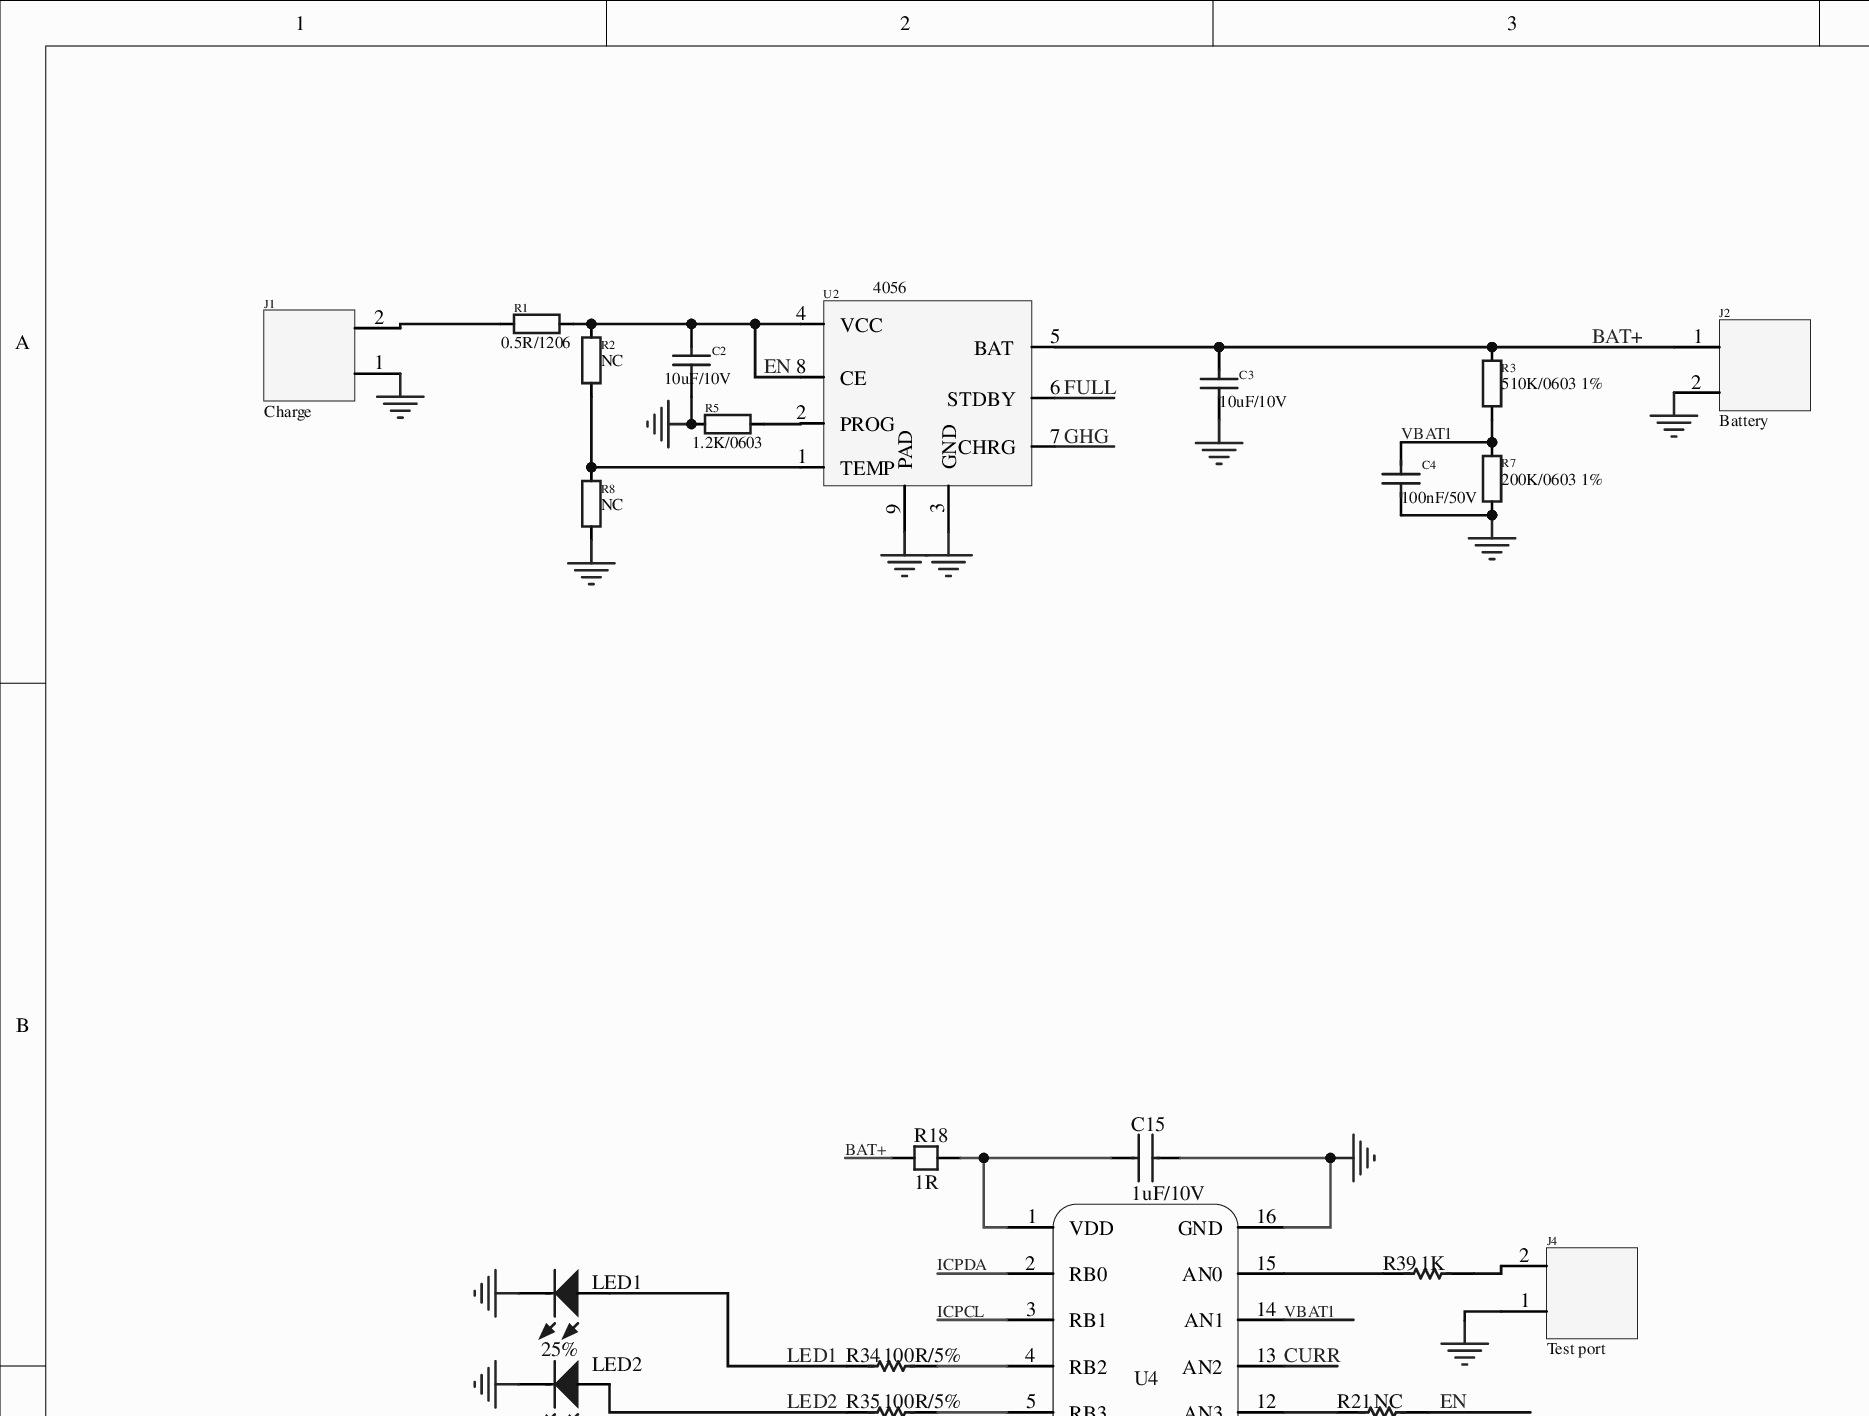
[diagram p0: MISC75737-5.SchDoc, top left]
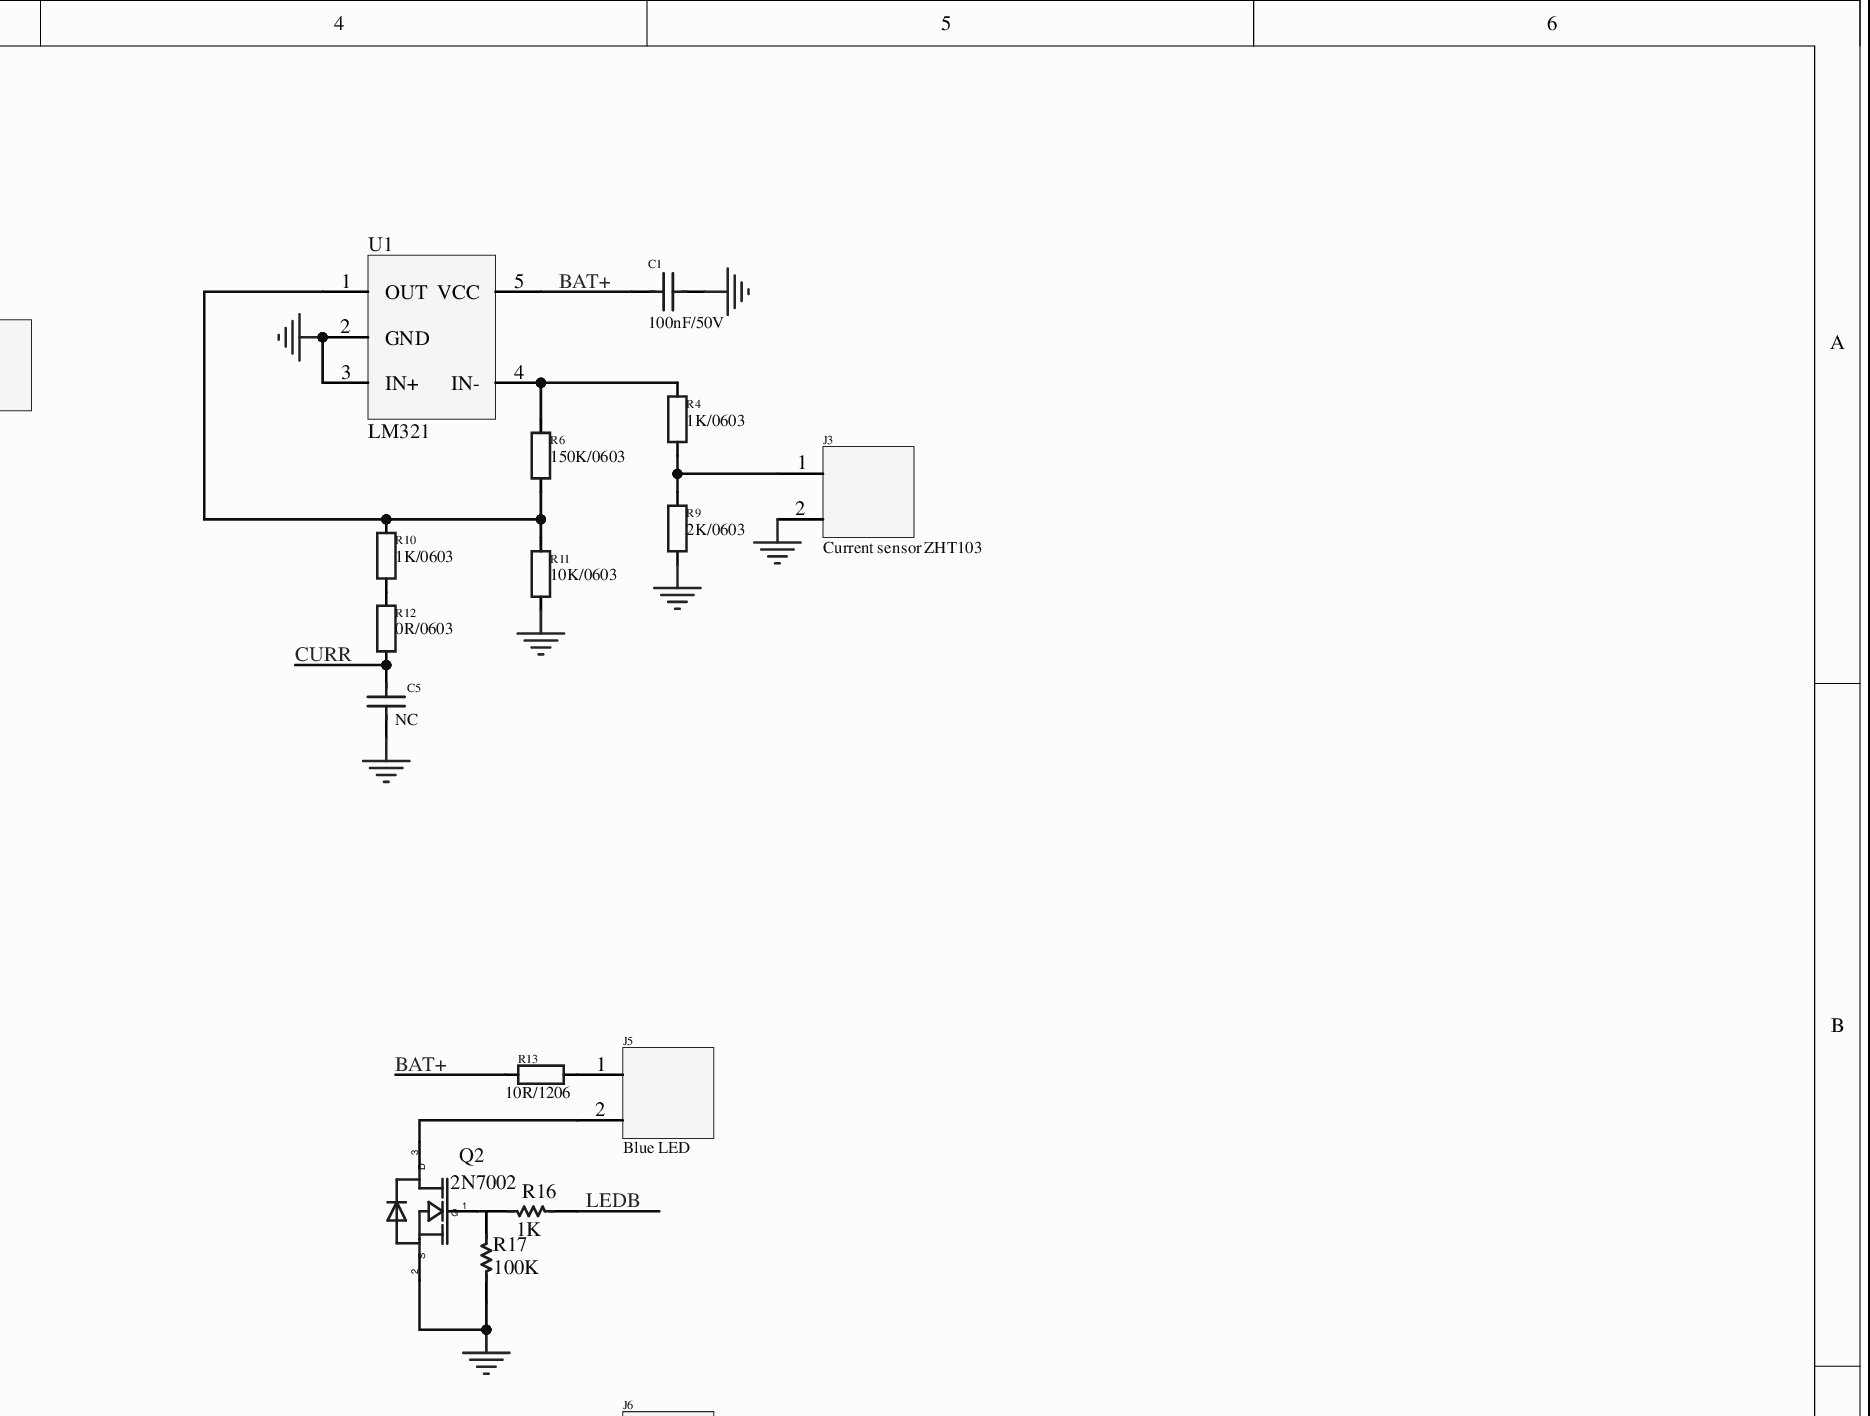
[diagram p1: MISC75737-5.SchDoc, top right]
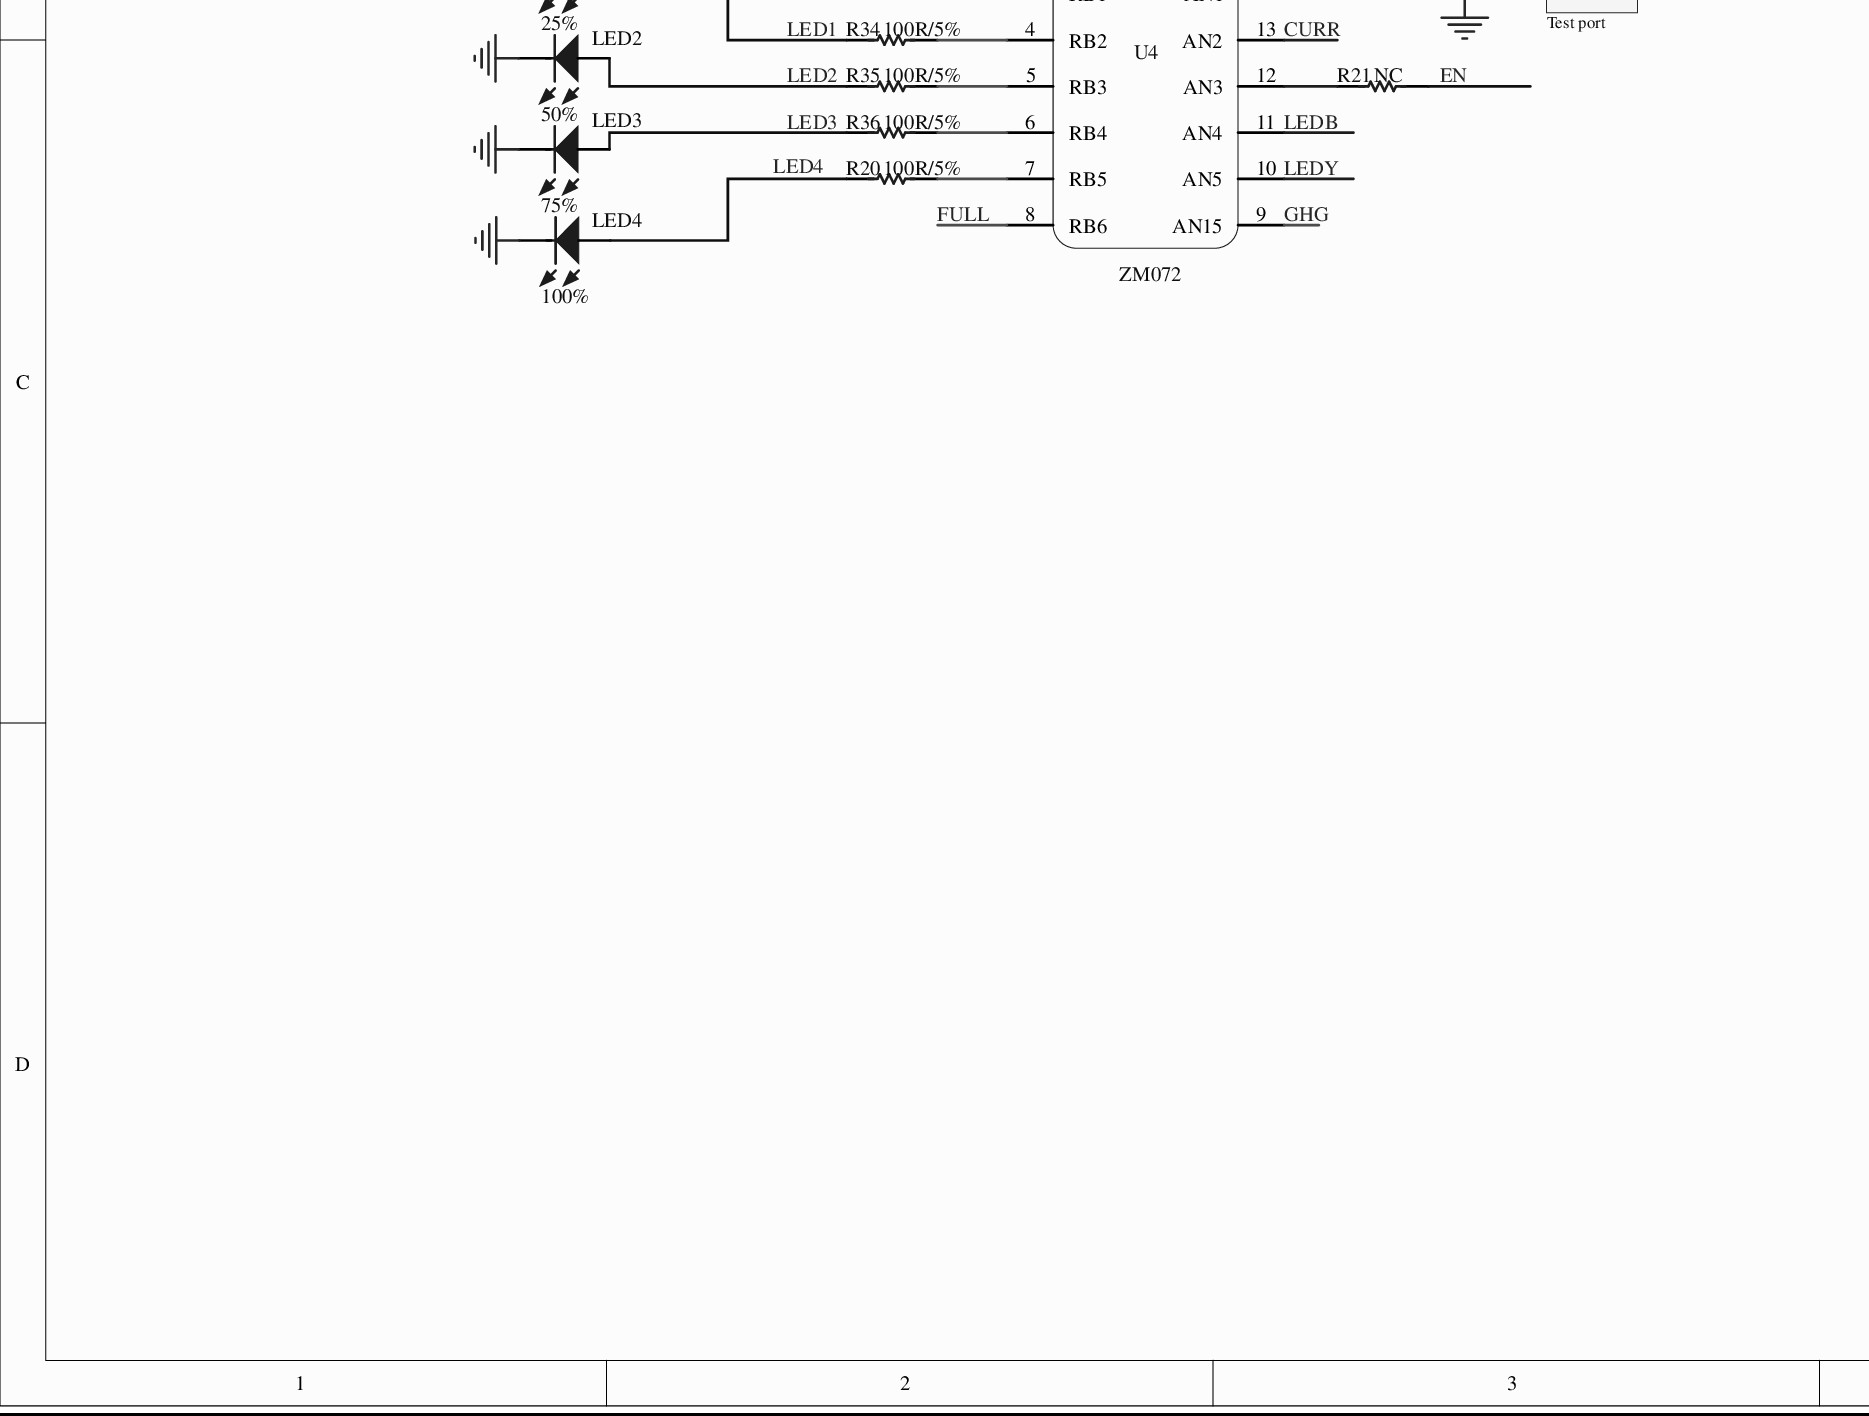
[diagram p2: MISC75737-5.SchDoc, bottom left]
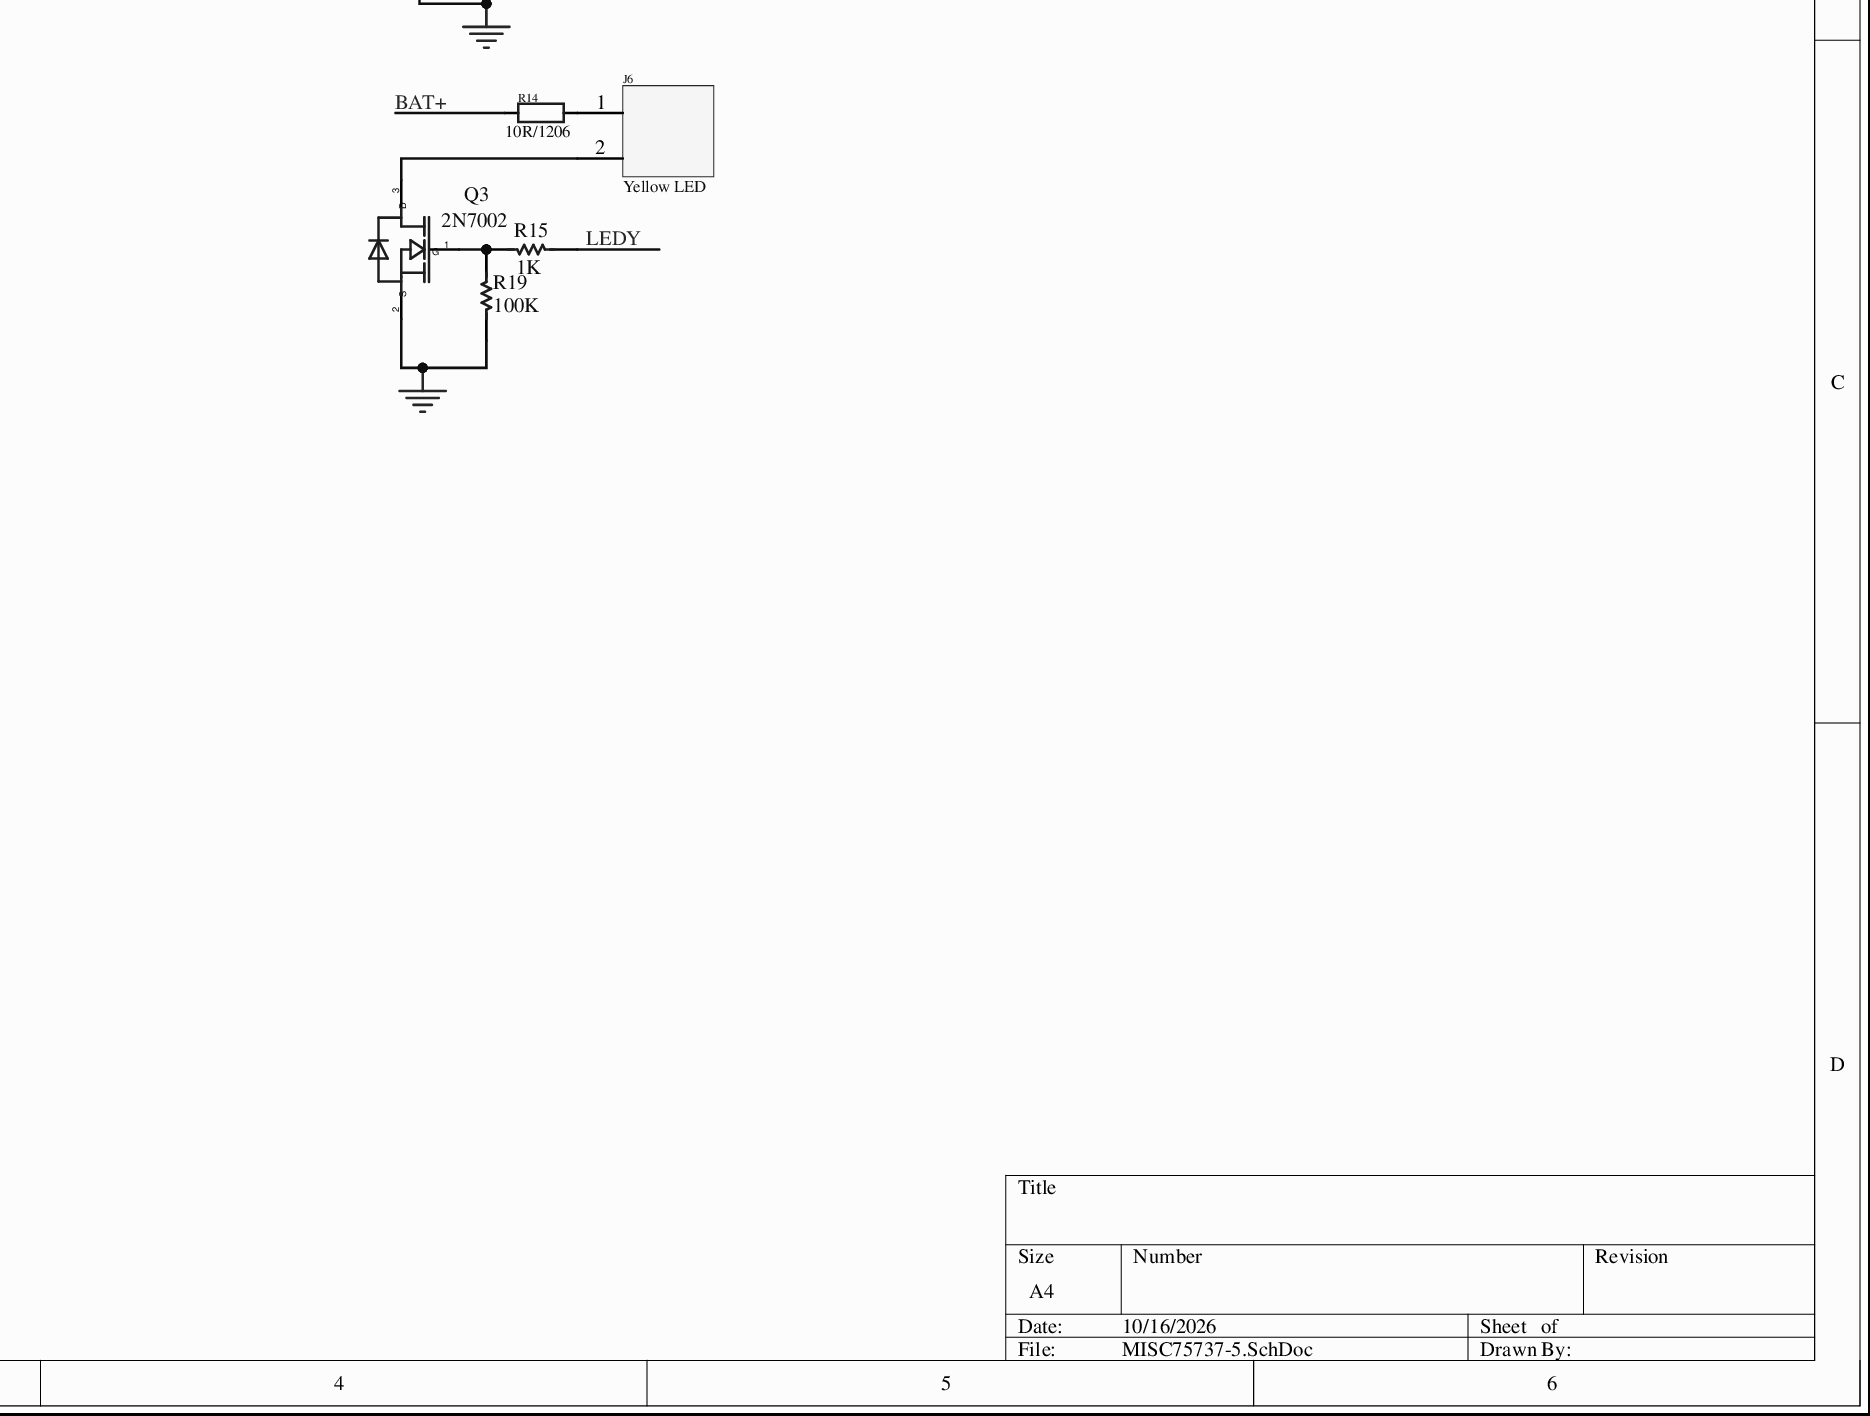
[diagram p3: MISC75737-5.SchDoc, bottom right]
# Altium project MISC75737-3.PrjPcb
1 sheet, 46 parts. Net scope: global (net labels, ports and power ports of the same name join across sheets).
Board file: MISC75737.PcbDoc

## Sheet MISC75737-5.SchDoc
size 400 x 299 mm; SheetNumber: 1; SheetTotal: 1

### Parts
C1  100nF/50V  [C0603A]
C2  10uF/10V  [C0805A]
C3  10uF/10V  [C0805A]
C4  100nF/50V  [C0603A]
C5  NC  [C0603A]
C15  1uF/10V  [C0603A]
J1  Charge  [HY2.0WT-2A/P 立贴带扣耐温260℃]
J2  Battery  [GH1.25-2PIN立贴带扣耐温260℃]
J3  Current sensor ZHT103  [IND-TH_L18.2-W10.2-P12.00-D0.9_ZHT103]
J4  Test port  [HY2.0WT-2A/P 立贴带扣耐温260℃]
J5  Blue LED  [GH1.25-2PIN立贴带扣耐温260℃]
J6  Yellow LED  [GH1.25-2PIN立贴带扣耐温260℃]
LED1  25%  [LED0603A]
LED2  50%  [LED0603A]
LED3  75%  [LED0603A]
LED4  100%  [LED0603A]
Q2  2N7002  [SOT23-3L]
Q3  2N7002  [SOT23-3L]
R1  0.5R/1206  [R1206A]
R2  NC  [R0603A]
R3  510K/0603 1%  [R0603A]
R4  1K/0603  [R0603A]
R5  1.2K/0603  [R0603A]
R6  150K/0603  [R0603A]
R7  200K/0603 1%  [R0603A]
R8  NC  [R0603A]
R9  2K/0603  [R0603A]
R10  1K/0603  [R0603A]
R11  10K/0603  [R0603A]
R12  0R/0603  [R0603A]
R13  10R/1206  [R1206A]
R14  10R/1206  [R1206A]
R15  1K  [R0603A]
R16  1K  [R0603A]
R17  100K  [R0603A]
R18  1R  [R0603A]
R19  100K  [R0603A]
R20  100R/5%  [R0603A]
R21  NC  [R0603A]
R34  100R/5%  [R0603A]
R35  100R/5%  [R0603A]
R36  100R/5%  [R0603A]
R39  1K  [R0603A]
U1  LM321  [SOT23-5A]
U2  4056  [ESOP-8L]
U4  ZM072  [SOP16L]

### Nets
GND: C1.1 C2.1 C3.1 C4.1 C5.1 C15.2 J1.1 J2.2 J3.2 J4.1 LED1.2 LED2.2 LED3.2 LED4.2 Q2.2(S) Q3.2(S) R5.1 R7.1 R8.1 R9.2 R11.2 R17.1 R19.1 U1.2(GND) U1.3(IN+) U2.3(GND) U2.9(PAD) U4.16(GND)
BAT+: C1.2 C3.2 J2.1 R3.2 R13.1 R14.1 R18.1 U1.5(VCC) U2.5(BAT)
CURR: C5.2 R12.2 U4.13(AN2)
EN: C2.2 R1.2 R2.2 R21.2 U2.4(VCC) U2.8(CE)
FULL: U2.6(STDBY) U4.8(RB6)
GHG: U2.7(CHRG) U4.9(AN15)
ICPCL: U4.3(RB1)
ICPDA: U4.2(RB0)
LED1: LED1.1 R34.1
LED2: LED2.1 R35.1
LED3: LED3.1 R36.1
LEDB: R16.2 U4.11(AN4)
LEDY: R15.2 U4.10(AN5)
VBAT1: C4.2 R3.1 R7.2 U4.14(AN1)
NetC15_1: C15.1 R18.2 U4.1(VDD)
NetJ1_2: J1.2 R1.1
NetJ3_1: J3.1 R4.2 R9.1
NetJ4_2: J4.2 R39.2
NetJ5_1: J5.1 R13.2
NetJ5_2: J5.2 Q2.3(D)
NetJ6_1: J6.1 R14.2
NetJ6_2: J6.2 Q3.3(D)
NetLED4_1: LED4.1 R20.1
NetQ2_1: Q2.1(G) R16.1 R17.2
NetQ3_1: Q3.1(G) R15.1 R19.2
NetR2_1: R2.1 R8.2 U2.1(TEMP)
NetR4_1: R4.1 R6.1 U1.4(IN-)
NetR5_2: R5.2 U2.2(PROG)
NetR6_2: R6.2 R10.1 R11.1 U1.1(OUT)
NetR10_2: R10.2 R12.1
NetR20_2: R20.2 U4.7(RB5)
NetR21_1: R21.1 U4.12(AN3)
NetR34_2: R34.2 U4.4(RB2)
NetR35_2: R35.2 U4.5(RB3)
NetR36_2: R36.2 U4.6(RB4)
NetR39_1: R39.1 U4.15(AN0)

### Notes on the sheet
- Labels drawn without touching a wire or pin: LED4

### Library data of the parts
C1 C4 C5 = Cap0603
C2 C3 = Cap0805: SMD capacitor; 规格: 0805-16V-106-X7R
C15 = CH
J1-J6 = 2PIN: DC socket right-angle 90° pitch 2.0; 物料名称: DC socket 2PIN; 封装: Pitch 2.0 90° right-angle THT
LED1-LED4 = LED 白发蓝: SMD LED; 规格: 0603-diffused-ice blue
Q2 Q3 = 2N7002: SMD MOS
R1 R13 R14 = Res1206: SMD resistor; 规格: 0603-43.2K-1%
R2-R12 R15-R17 R19-R21 R34-R36 R39 = Res0603: SMD resistor; 规格: 0603
R18 = RH1
U2 = TP4056: Charger IC; 规格: ESOP-8; 物料名称: Charger IC 4056
U4 = MCU-TSSOP-16